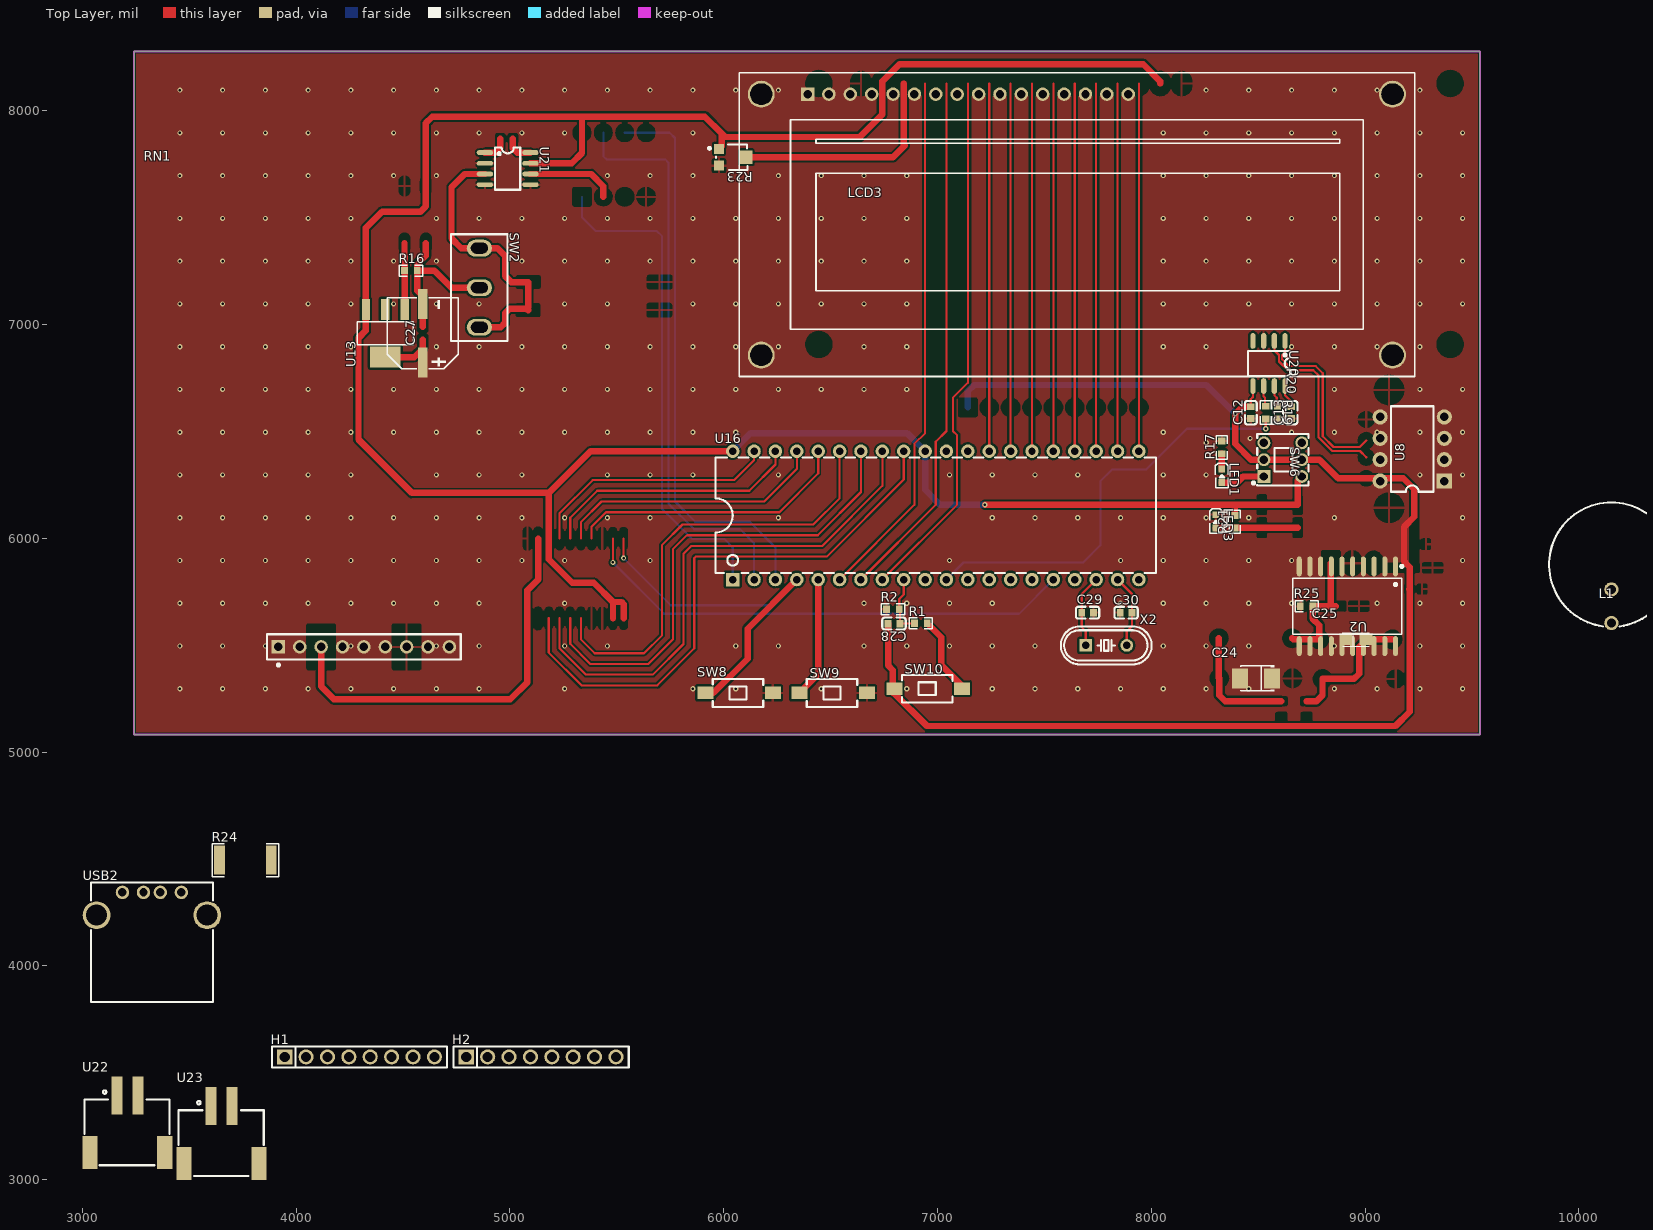
[diagram p0: Top Layer view]
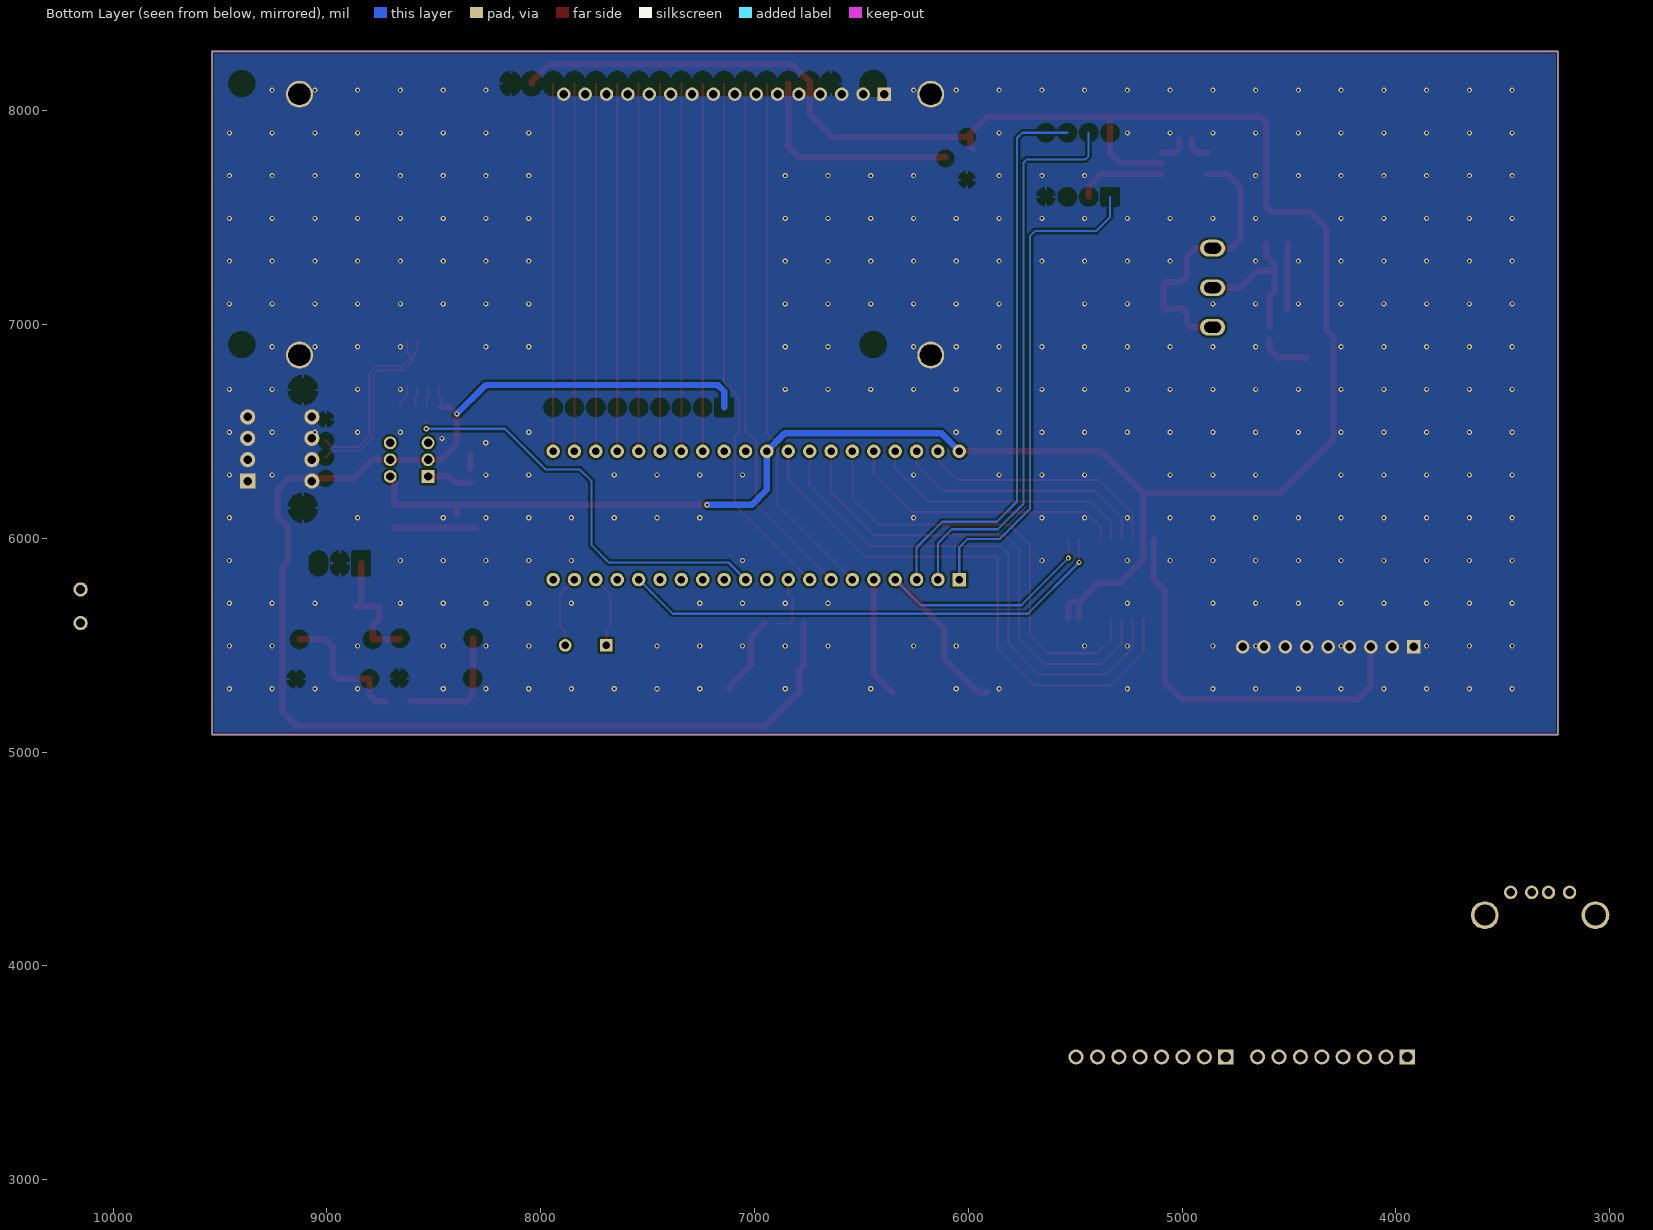
[diagram p1: Bottom Layer view, seen from below]
# Altium PCB MISC52088.pcbdoc
Units mil, origin at the board's own origin, x right, y up, seen from the top; angles counter-clockwise.
Board outline 6295 x 3195 mil, 2 copper layers (Top Layer, Bottom Layer), stack 62.206 mil thick; 40 components, 56 nets, 207 pads, 333 vias.

## Layer stack, top to bottom
Top Solder Mask Layer: solder mask 0.394, Dk 3.3
Top Layer: signal copper 1.379
Dielectric1: surface 59.449, FR4, Dk 4.5
Bottom Layer: signal copper 1.378
Bottom Solder Mask Layer: solder mask 0.394, Dk 3.3

## Board outline
3242.1,8277.43 3242.1,5082.43 9537.1,5082.43 9537.1,8277.43

## Design rules (kind name [scope] priority, off if disabled: settings)
BoardOutlineClearance copperThickness2oz_1 [All] p2 off: genericclearance=7.99 ignorepadtopadclearanceinfootprint=FALSE except(0: Arc-SplitContinuation Track-SplitContinuation SMDPad-SplitContinuation THPad-SplitContinuation Via-SplitContinuation Fill-SplitContinuation Region-SplitContinuation Poly-SplitContinuation Text-SplitContinuation Hole-SplitContinuation; 5.98: Arc-OutlineEdge Track-OutlineEdge SMDPad-OutlineEdge THPad-OutlineEdge Via-OutlineEdge Fill-OutlineEdge Region-OutlineEdge Text-OutlineEdge Hole-OutlineEdge SMDPad-CutoutEdge THPad-CutoutEdge Via-CutoutEdge Fill-CutoutEdge Region-CutoutEdge Text-CutoutEdge Hole-CutoutEdge; 10: Poly-OutlineEdge Poly-CutoutEdge; 11.81: Arc-CutoutEdge Track-CutoutEdge)
BoardOutlineClearance Plane_innerPlane_1 [All] p4 off: genericclearance=4.02 ignorepadtopadclearanceinfootprint=FALSE except(0: Arc-SplitContinuation Track-SplitContinuation SMDPad-SplitContinuation THPad-SplitContinuation Via-SplitContinuation Fill-SplitContinuation Region-SplitContinuation Poly-SplitContinuation Text-SplitContinuation Hole-SplitContinuation; 5.98: Arc-OutlineEdge Track-OutlineEdge SMDPad-OutlineEdge THPad-OutlineEdge Via-OutlineEdge Fill-OutlineEdge Region-OutlineEdge Text-OutlineEdge Hole-OutlineEdge SMDPad-CutoutEdge THPad-CutoutEdge Via-CutoutEdge Fill-CutoutEdge Region-CutoutEdge Text-CutoutEdge Hole-CutoutEdge; 10: Poly-OutlineEdge Poly-CutoutEdge; 11.81: Arc-CutoutEdge Track-CutoutEdge)
BoardOutlineClearance Copper_copperRegion_1 [All] p6 off: genericclearance=4.02 ignorepadtopadclearanceinfootprint=FALSE except(0: Arc-SplitContinuation Track-SplitContinuation SMDPad-SplitContinuation THPad-SplitContinuation Via-SplitContinuation Fill-SplitContinuation Region-SplitContinuation Poly-SplitContinuation Text-SplitContinuation Hole-SplitContinuation; 5.98: Arc-OutlineEdge Track-OutlineEdge SMDPad-OutlineEdge THPad-OutlineEdge Via-OutlineEdge Fill-OutlineEdge Region-OutlineEdge Text-OutlineEdge Hole-OutlineEdge SMDPad-CutoutEdge THPad-CutoutEdge Via-CutoutEdge Fill-CutoutEdge Region-CutoutEdge Text-CutoutEdge Hole-CutoutEdge; 10: Poly-OutlineEdge Poly-CutoutEdge; 11.81: Arc-CutoutEdge Track-CutoutEdge)
BoardOutlineClearance copperThickness1oz_1 [All] p8: genericclearance=4.02 ignorepadtopadclearanceinfootprint=FALSE except(0: Arc-SplitContinuation Track-SplitContinuation SMDPad-SplitContinuation THPad-SplitContinuation Via-SplitContinuation Fill-SplitContinuation Region-SplitContinuation Poly-SplitContinuation Text-SplitContinuation Hole-SplitContinuation; 5.98: Arc-OutlineEdge Track-OutlineEdge SMDPad-OutlineEdge THPad-OutlineEdge Via-OutlineEdge Fill-OutlineEdge Region-OutlineEdge Text-OutlineEdge Hole-OutlineEdge SMDPad-CutoutEdge THPad-CutoutEdge Via-CutoutEdge Fill-CutoutEdge Region-CutoutEdge Text-CutoutEdge Hole-CutoutEdge; 10: Poly-OutlineEdge Poly-CutoutEdge; 11.81: Arc-CutoutEdge Track-CutoutEdge)
Clearance copperThickness2oz [All] p1 off: gap=7.99 ignorepadtopadclearanceinfootprint=FALSE except(5.98: SMDPad-Track SMDPad-SMDPad THPad-Track SMDPad-THPad THPad-THPad Track-Via SMDPad-Via THPad-Via Via-Via Fill-Track Region-Track Fill-SMDPad Region-SMDPad Fill-THPad Region-THPad Fill-Via Region-Via Fill-Fill Fill-Region Region-Region Arc-SMDPad Arc-THPad Arc-Via Fill-Arc Region-Arc Arc-Arc Text-Track SMDPad-Text Text-THPad Text-Via Fill-Text Region-Text Text-Text Hole-Track Hole-SMDPad Hole-THPad Hole-Via Fill-Hole Region-Hole Hole-Arc Hole-Text; 10: Poly-Track Poly-SMDPad Poly-THPad Poly-Via Poly-Fill Poly-Region Poly-Poly Poly-Arc Poly-Text Poly-Hole; 11.81: Arc-Track Arc-Text)
Clearance Plane_innerPlane [All] p3 off: gap=4.02 ignorepadtopadclearanceinfootprint=FALSE except(5.98: SMDPad-Track SMDPad-SMDPad THPad-Track SMDPad-THPad THPad-THPad Track-Via SMDPad-Via THPad-Via Via-Via Fill-Track Region-Track Fill-SMDPad Region-SMDPad Fill-THPad Region-THPad Fill-Via Region-Via Fill-Fill Fill-Region Region-Region Arc-SMDPad Arc-THPad Arc-Via Fill-Arc Region-Arc Arc-Arc Text-Track SMDPad-Text Text-THPad Text-Via Fill-Text Region-Text Text-Text Hole-Track Hole-SMDPad Hole-THPad Hole-Via Fill-Hole Region-Hole Hole-Arc Hole-Text; 10: Poly-Track Poly-SMDPad Poly-THPad Poly-Via Poly-Fill Poly-Region Poly-Poly Poly-Arc Poly-Text Poly-Hole; 11.81: Arc-Track Arc-Text)
Clearance Copper_copperRegion [All] p5 off: gap=4.02 ignorepadtopadclearanceinfootprint=FALSE except(5.98: SMDPad-Track SMDPad-SMDPad THPad-Track SMDPad-THPad THPad-THPad Track-Via SMDPad-Via THPad-Via Via-Via Fill-Track Region-Track Fill-SMDPad Region-SMDPad Fill-THPad Region-THPad Fill-Via Region-Via Fill-Fill Fill-Region Region-Region Arc-SMDPad Arc-THPad Arc-Via Fill-Arc Region-Arc Arc-Arc Text-Track SMDPad-Text Text-THPad Text-Via Fill-Text Region-Text Text-Text Hole-Track Hole-SMDPad Hole-THPad Hole-Via Fill-Hole Region-Hole Hole-Arc Hole-Text; 10: Poly-Track Poly-SMDPad Poly-THPad Poly-Via Poly-Fill Poly-Region Poly-Poly Poly-Arc Poly-Text Poly-Hole; 11.81: Arc-Track Arc-Text)
Clearance copperThickness1oz [All] p7: gap=4.02 ignorepadtopadclearanceinfootprint=FALSE except(5.98: SMDPad-Track SMDPad-SMDPad THPad-Track SMDPad-THPad THPad-THPad Track-Via SMDPad-Via THPad-Via Via-Via Fill-Track Region-Track Fill-SMDPad Region-SMDPad Fill-THPad Region-THPad Fill-Via Region-Via Fill-Fill Fill-Region Region-Region Arc-SMDPad Arc-THPad Arc-Via Fill-Arc Region-Arc Arc-Arc Text-Track SMDPad-Text Text-THPad Text-Via Fill-Text Region-Text Text-Text Hole-Track Hole-SMDPad Hole-THPad Hole-Via Fill-Hole Region-Hole Hole-Arc Hole-Text; 10: Poly-Track Poly-SMDPad Poly-THPad Poly-Via Poly-Fill Poly-Region Poly-Poly Poly-Arc Poly-Text Poly-Hole; 11.81: Arc-Track Arc-Text)
DiffPairsRouting differentialPair [All] p1: maxlimit=6 minlimit=6 mostfreqgap=6 toplayer_minwidth=5 toplayer_prefwidth=10 toplayer_maxwidth=100 toplayer_mingap=6 toplayer_prefgap=6 toplayer_maxgap=6 bottomlayer_minwidth=5 bottomlayer_prefwidth=10 bottomlayer_maxwidth=100 bottomlayer_mingap=6 bottomlayer_prefgap=6 bottomlayer_maxgap=6 maxuncoupledlength=10
HoleToHoleClearance otherClearance [All] p1: gap=11.8 allowstackedmicrovias=TRUE
Length netLength [All] p1: minlimit=0 maxlimit=0
PasteMaskExpansion pasteMaskExpansion [All] p1: expansion=0
PlaneConnect innerPlane [All] p1: planeconnectstyle=Relief reliefexpansion=20 reliefentries=4 reliefconductorwidth=10 reliefairgap=10
PolygonConnect copperRegion [All] p1: connectstyle=Relief reliefconductorwidth=10 reliefentries=4 polygonreliefangle="90 Angle" airgapwidth=10 via.connectstyle=Relief via.reliefconductorwidth=10 via.reliefentries=4 via.polygonreliefangle="90 Angle" via.airgapwidth=10
RoutingVias viaSize [All] p1: holewidth=12.01 width=24.02 viastyle="Through Hole" minholewidth=11.81 minwidth=19.68 maxholewidth=248.03 maxwidth=393.7
SolderMaskExpansion solderMaskExpansion [IsVia] p1: expansion=-1000 istentingtop=TRUE
SolderMaskExpansion solderMaskExpansion [All] p2: expansion=2 istentingtop=FALSE
Width copperThickness2oz_2 [All] p1 off: maxlimit=100 minlimit=8 preferedwidth=10
Width copperThickness1oz_2 [All] p2: maxlimit=100 minlimit=5 preferedwidth=10

## Components (designator, comment, footprint, x,y, rotation, side; value= is the part's Value field where it differs from the comment)
C12 "0.1uF" C0603 8465.54,6587.96 r90 top
C13 "0.1uF" C0603 8655.54,6588.08 r90 top
C24 "22uF" CAP-SMD_L3.5-W2.8-R-RD 8489.27,5345.01 r0 top
C25 "100nF" CASE-A_3216 8957.1,5527.43 r0 top
C27 "100uF" CAP-SMD_BD8.1-L8.3-W8.3-LS9.3-FD 4592.12,6959.41 r90 top
C28 "47pF" C0603 6796.59,5601.57 r180 top
C29 "47pF" C0603 7702.1,5652.43 r180 top
C30 "10uF" C0603 7882.1,5652.43 r0 top
H1 "" HDR-TH_8P-P2.54-V-F-1 4296.74,3574.67 r0 top
H2 "" HDR-TH_8P-P2.54-V-F-1 5146.11,3574.67 r0 top
L1 "22uH" IND-TH_BD14.7-2P-P4.00 10152.1,5682.43 r0 top
LCD3 "HS1602A" LCD1602 7652.1,7467.43 r0 top
LED1 "" LED_0603 8330.05,6290.49 r270 top
LED3 "" LED_0603 8302.1,6077.43 r270 top
R1 "10K" R0603 6922.1,5602.43 r0 top
R2 "10K" R0603 6791.31,5668.48 r0 top
R16 "100K" R0603 4537.1,7252.43 r0 top
R17 "1K" R0603 8330.05,6425.24 r90 top
R19 "100Ω" R0603 8590.54,6588.08 r270 top
R20 "100Ω" R0603 8535.54,6588.08 r270 top
R21 "1K" R0603 8391.2,6077.73 r90 top
R23 "10kΩ" RES-ADJ-SMD_3P-L3.0-W3.8-P1.75-BR 6042.1,7782.43 r180 top
R24 "5Ω" R2512 3763,4495.45 r0 top
R25 "14kΩ" R0603 8726.82,5682.13 r0 top
RN1 "1kΩ" RES-ARRAY-TH_9P-P2.54-D1.0 4317.1,5492.43 r0 top
SW2 "SS-12D10L5" SW-TH_SS-12D10L5 4857.1,7172.43 r270 top
SW6 "5.8 ZSGT" SW-TH_5.8ZSGT 8615.54,6367.97 r270 top
SW8 "TS-1101-C-W" SW-SMD_L6.0-W3.3-LS8.0 6072.1,5277.43 r0 top
SW9 "TS-1101-C-W" SW-SMD_L6.0-W3.3-LS8.0 6512.1,5277.43 r0 top
SW10 "TS-1101-C-W" SW-SMD_L6.0-W3.3-LS8.0 6957.1,5297.43 r0 top
U2 "DAC0832LCWMX/NOPB" SOIC-20_L13.0-W7.6-P1.27-LS10.3-BL 8917.1,5682.43 r180 top
U8 "ADC0832CCN" DIP-8_L9.7-W6.4-P2.54-LS7.6-BL 9220.54,6417.97 r90 top
U13 "LT3092EST#TRPBF" SOT-223-4_L6.5-W3.5-P2.30-LS7.0-BR 4417.12,6959.41 r90 top
U16 "STC89C52RC-40I-PDIP40" DIP-40_L52.0-W13.7-P2.54-LS15.2-BL 6992.1,6107.43 r0 top
U20 "CH340N" SOP-8_L4.9-W3.9-P1.27-LS6.0-BL 8550.54,6817.97 r180 top
U21 "AD620ARZ-REEL7" SOIC-8_L5.0-W4.0-P1.27-LS6.0-BL 4989.7,7729.25 r270 top
U22 "XH2.54-2PSMD" CONN-SMD_XH2.54-2PSMD 3210.63,3260.63 r0 top
U23 "XH2.54-2PSMD" CONN-SMD_XH2.54-2PSMD 3651.58,3210.63 r0 top
USB2 "USB-231-ARY" USB-A-TH_USB-231-ARY 3325.62,4290.73 r0 top
X2 "11.0592MHz" HC-49US_L11.5-W4.5-P4.88 7789.27,5499.25 r0 top

## Footprints (in the part's own frame and the unit in brackets; to place one, negate y for a bottom-side part, rotate by r counter-clockwise, add the part's x,y. Pads: shape width x height; smd on the part's side, far side on the other; paste and mask are expansions set on the pad)
C0603 [mm]
  rect 0.8x0.9 smd: 1(-0.7,0) 2(0.7,0)
  silkscreen extent -1.39,-0.71 1.39,0.71
CAP-SMD_BD8.1-L8.3-W8.3-LS9.3-FD [mm]
  rect 3.56x1.12 smd: 1(-3.47,0) 2(3.47,0)
  silkscreen extent -4.23,-4.23 4.23,4.23
CAP-SMD_L3.5-W2.8-R-RD [mm]
  rect 1.9x2.376 smd: 1(1.899,0) 2(-1.899,0)
  silkscreen extent -1.83,-1.55 2.21,1.55
CASE-A_3216 [mil]
  rect 59.05x53.5 smd: 1(-47.24,0) 2(47.24,0)
  silkscreen extent -63,-32 63,32
CONN-SMD_XH2.54-2PSMD [mm]
  rect 1.3x4.5 smd paste+0 mask+0.05: 1(-1.25,3.4) 2(1.25,3.4)
  rect 1.8x3.9 smd paste+0 mask+0.05: 3(-4.45,-3.4) 4(4.45,-3.4)
  silkscreen extent -5.1,-4.9 5,4
DIP-8_L9.7-W6.4-P2.54-LS7.6-BL [mm]
  rect 1.8x1.8 hole 1 paste+0 mask+0.05: 1(-3.81,-3.81)
  round 1.8 hole 1 paste+0 mask+0.05: 2(-1.27,-3.81) 3(1.27,-3.81) 4(3.81,-3.81) 5(3.81,3.81) 6(1.27,3.81) 7(-1.27,3.81) 8(-3.81,3.81)
  silkscreen extent -5.08,-2.53 5.08,2.53
DIP-40_L52.0-W13.7-P2.54-LS15.2-BL [mil]
  rect 63x63 hole 35: 1(-950,-300)
  round 63 hole 35: 2(-850,-300) 3(-750,-300) 4(-650,-300) 5(-550,-300) 6(-450,-300) 7(-350,-300) 8(-250,-300) 9(-150,-300) 10(-50,-300) 11(50,-300) 12(150,-300) 13(250,-300) 14(350,-300) 15(450,-300) 16(550,-300) 17(650,-300) 18(750,-300) 19(850,-300) 20(950,-300) 21(950,300) 22(850,300) 23(750,300) 24(650,300) 25(550,300) 26(450,300) 27(350,300) 28(250,300) 29(150,300) 30(50,300) 31(-50,300) 32(-150,300) 33(-250,300) 34(-350,300) 35(-450,300) 36(-550,300) 37(-650,300) 38(-750,300) 39(-850,300) 40(-950,300)
  silkscreen extent -1030,-270 1030,270
HC-49US_L11.5-W4.5-P4.88 [mm]
  rect 1.5x1.5 hole 0.9: 1(-2.44,0)
  round 1.5 hole 0.9: 2(2.44,0)
  silkscreen extent -5.39,-2.25 5.39,2.25
HDR-TH_8P-P2.54-V-F-1 [mm]
  rect 1.8x1.8 hole 1.2: 1(-8.89,0)
  round 1.8 hole 1.2: 2(-6.35,0) 3(-3.81,0) 4(-1.27,0) 5(1.27,0) 6(3.81,0) 7(6.35,0) 8(8.89,0)
  silkscreen extent -10.41,-1.25 10.41,1.25
IND-TH_BD14.7-2P-P4.00 [mm]
  round 1.7 hole 1.1 paste+0 mask+0.05: 1(0,-2) 2(0,2)
  silkscreen extent -7.4,-2.39 7.4,12.35
LCD1602 [mm]
  round 3.2 hole 2.5 slot 2.625 at 0 deg: 0(-37.5,-15.5) 0(-37.5,15.5) 0(37.5,-15.5) 0(37.5,15.5)
  rect 1.6x1.6 hole 1: 1(-32,15.5)
  round 1.6 hole 1: 2(-29.46,15.5) 3(-26.92,15.5) 4(-24.38,15.5) 5(-21.84,15.5) 6(-19.3,15.5) 7(-16.76,15.5) 8(-14.22,15.5) 9(-11.68,15.5) 10(-9.14,15.5) 11(-6.6,15.5) 12(-4.06,15.5) 13(-1.52,15.5) 14(1.02,15.5) 15(3.56,15.5) 16(6.1,15.5)
  silkscreen extent -40.13,-18.03 40.13,18.03
LED_0603 [mil]
  rect 31.5x31.5 smd paste+0 mask+2: 1(-33.5,-0.4) 2(29.5,-0.2)
  silkscreen extent -61,-30 53,30
R0603 [mil]
  rect 31.75x34.02 smd paste-3937.01 mask+2: 1(-29.66,0) 2(29.66,0)
  silkscreen extent -55,-26 55,26
R2512 [mil]
  rect 50.49x136.06 smd paste-3937.01 mask+2: 1(-120.72,0) 2(120.72,0)
  silkscreen extent -155,-77 155,77
RES-ADJ-SMD_3P-L3.0-W3.8-P1.75-BR [mm]
  rect 1.2x1.2 smd: 1(1.625,-1) 3(1.625,1)
  rect 1.5x1.6 smd: 2(-1.625,0)
  silkscreen extent -1.75,-1.51 2.92,1.51
RES-ARRAY-TH_9P-P2.54-D1.0 [mm]
  rect 1.6x1.6 hole 1: 1(-10.16,0)
  round 1.6 hole 1: 2(-7.62,0) 3(-5.08,0) 4(-2.54,0) 5(0,0) 6(2.54,0) 7(5.08,0) 8(7.62,0) 9(10.16,0)
  silkscreen extent -11.5,-2.31 11.5,1.5
SOIC-8_L5.0-W4.0-P1.27-LS6.0-BL [mil]
  oval 22.38x76.78 smd: 1(-75,-106.5) 2(-25,-106.5) 3(25,-106.5) 4(75,-106.5) 5(75,106.5) 6(25,106.5) 7(-25,106.5) 8(-75,106.5)
  silkscreen extent -98,-59 98,59
SOIC-20_L13.0-W7.6-P1.27-LS10.3-BL [mm]
  oval 0.595x2.36 smd: 1(-5.715,-4.73) 2(-4.445,-4.73) 3(-3.175,-4.73) 4(-1.905,-4.73) 5(-0.635,-4.73) 6(0.635,-4.73) 7(1.905,-4.73) 8(3.175,-4.73) 9(4.445,-4.73) 10(5.715,-4.73) 11(5.715,4.73) 12(4.445,4.73) 13(3.175,4.73) 14(1.905,4.73) 15(0.635,4.73) 16(-0.635,4.73) 17(-1.905,4.73) 18(-3.175,4.73) 19(-4.445,4.73) 20(-5.715,4.73)
  silkscreen extent -6.61,-4.88 6.48,3.32
SOP-8_L4.9-W3.9-P1.27-LS6.0-BL [mm]
  oval 0.63x1.865 smd: 1(-1.905,-2.682) 2(-0.635,-2.682) 3(0.635,-2.682) 4(1.905,-2.682) 5(1.905,2.682) 6(0.635,2.682) 7(-0.635,2.682) 8(-1.905,2.682)
  silkscreen extent -2.5,-1.5 2.5,1.48
SOT-223-4_L6.5-W3.5-P2.30-LS7.0-BR [mm]
  rect 2.47x0.98 smd: 1(2.835,-2.3) 2(2.835,0) 3(2.835,2.3)
  rect 2.47x3.6 smd: 4(-2.835,0)
  silkscreen extent -1.37,-3.33 1.37,3.33
SW-SMD_L6.0-W3.3-LS8.0 [mm]
  rect 1.9x1.5 smd: 1(-4,0) 2(4,0)
  silkscreen extent -3.14,-1.67 2.86,1.63
SW-TH_5.8ZSGT [mm]
  rect 1.524x1.524 hole 1: 1(2,-2.25)
  round 1.524 hole 1: 2(0,-2.25) 3(-2,-2.25) 4(2,2.25) 5(0,2.25) 6(-2,2.25)
  silkscreen extent -3.05,-3.64 3.05,3.05
SW-TH_SS-12D10L5 [mm]
  oval 2x3 hole 1.3 slot 2 at 90 deg: 1(-4.7,0) 2(0,0) 3(4.7,0)
  silkscreen extent -6.35,-3.35 6.35,3.35
USB-A-TH_USB-231-ARY [mm]
  round 1.6 hole 1: 1(-3.5,1.355) 2(-1,1.355) 3(1,1.355) 4(3.5,1.355)
  round 3.3 hole 2.5: 5(-6.57,-1.355) 6(6.57,-1.355)
  silkscreen extent -7.23,-11.68 7.24,2.54

## Via types
v1: diameter 24.02, hole 12, Top Layer to Bottom Layer, 333 vias

## Nets (pads, with @x,y where several pads share a name; then routed paths per layer and width w, separated by ;. In a path a pad name is that pad's centre, name@x,y a point inside that pad or via, vN(x,y) a via of type N, cw(c..) or ccw(c..) an arc to the next point about the centre after c; other vN are vias at no path point)
5V: LED1.2 SW6.1 U23.1 | length 208.8
  Top Layer w30: LED1.2 8400.66,6260.99 8428.89,6289.23 SW6.1
$1N1971: R1.2 SW10.2 | length 372.4
  Top Layer w30: R1.2 7017.1,5537.09 7017.1,5407.43 7114.58,5309.95 SW10.2
$1N7746: LCD3.7 RN1.2 U16.28 | length 1720
  Top Layer w10: U16.28 7242.1,8127.43
$1N7754: LCD3.8 RN1.3 U16.27 | length 1720
  Top Layer w10: U16.27 7342.1,8127.43
$1N7769: LCD3.9 RN1.4 U16.26 | length 1720
  Top Layer w10: U16.26 7442.1,8127.43
$1N7777: LCD3.10 RN1.5 U16.25 | length 1720
  Top Layer w10: U16.25 7542.1,8127.43
$1N7792: LCD3.11 RN1.6 U16.24 | length 1720
  Top Layer w10: U16.24 7642.1,8127.43
$1N7807: LCD3.12 RN1.7 U16.23 | length 1720
  Top Layer w10: U16.23 7742.1,8127.43
$1N7815: LCD3.13 RN1.8 U16.22 | length 1720
  Top Layer w10: U16.22 7842.1,8127.43
$1N7830: LCD3.14 RN1.9 U16.21 | length 1720
  Top Layer w10: U16.21 7942.1,8127.43
$1N9685: C30.1 R1.1 R2.2 U16.9 | length 284.6
  Top Layer w10: U16.9 6842.1,5737.43 6820.97,5716.3 R2.2 6824.15,5665.3 6824.15,5601.57 6891.57,5601.57 R1.1
$1N13806:  | length 639.9
  Top Layer w30: 8726.16,5238.26 8772.93,5238.26 8800.84,5266.17 8800.84,5342.43 8947.1,5342.43 8972.1,5367.43 8972.1,5492.43 9007.1,5527.43 9128.36,5527.43
$1N14180:  | length 568.6
  Top Layer w30: 8315.84,5532.43 8315.84,5347.18 8318.01,5345.01 8318.01,5266.52 8346.27,5238.26 8608.05,5238.26
$1N17500: R24.1 U13.4 | length 233.7
  Top Layer w30: U13.4 4552.47,6847.8 4592.12,6887.46 4592.12,6929.75
$1N18707: C28.2 U16.18 X2.1 | length 343.9
  Top Layer w10: X2.1 7693.22,5566.32 7674.54,5584.99 7674.54,5652.43 7674.54,5739.87 U16.18
$1N18717: C29.2 U16.19 X2.2 | length 346.2
  Top Layer w10: U16.19 7909.66,5739.87 7909.66,5652.43 7909.66,5589.99 7885.34,5565.67 X2.2
$1N19281:  | length 606.9
  Top Layer w30: 8658.36,5532.43 8663.36,5527.43 8785.84,5527.43 8785.84,5593.69 8754.38,5625.16 8754.38,5682.13 8755.23,5682.98 8839.29,5682.98 ; 8839.93,5883.36 8839.93,5683.62 8839.29,5682.98 ; 8863,5682.98 8839.29,5682.98
$1N20482: R16.1 U13.1 | length 309.8
  Top Layer w30: 4507.12,7380.55 4507.12,7317.41 4507.44,7317.09 R16.1 4507.44,7158.24 4507.67,7158.01 U13.1
$1N25075: LED1.1 R17.1 | length 71.8
  Top Layer w30: LED1.1 8330.05,6324.39 R17.1
$1N27445: LCD3.3 R23.2 | length 1055.9
  Top Layer w30: R23.2 6792.1,7782.43 6847.1,7837.43 6842.1,7842.43 6842.1,8127.43
$1N30925: C13.2 U20.8 | length 109.1
  Top Layer w10: U20.8 8625.54,6668.99 8655.54,6638.99 C13.2
$1N30929: R19.1 U20.7 | length 100.8
  Top Layer w10: U20.7 8575.54,6668.99 8587.1,6657.43 8587.1,6621.19 R19.1
$1N30932: R20.1 U20.6 | length 98.8
  Top Layer w10: U20.6 8525.54,6663.99 8532.1,6657.43 8532.1,6621.19 R20.1
$1N33023:  | length 383
  Top Layer w30: 8301.9,6047.93 8303.52,6049.55 8684.28,6049.55
$1N35283: R16.2 R24.2 SW2.2 | length 731.8
  Top Layer w30: R16.2@4577.1,7252.43 4647.1,7252.43 4727.1,7172.43 SW2.2 ; 4592.12,6989.07 4592.12,7132.41 4566.76,7157.77 R16.2 4566.76,7282.09 4607.12,7322.46 4607.12,7380.55
$1N38066: R25.2 U21.1 | length 124.5
  Top Layer w30: U21.1 4933.92,7804.25 4955.04,7825.37 4955.04,7869.25
$1N38070: R25.1 U21.8 | length 134.6
  Top Layer w30: 5014.36,7869.25 5014.36,7825.17 5035.28,7804.25 U21.8
$1N38159: H1.1 H2.1 SW2.1 SW2.3 U21.3 | length 1341.7
  Top Layer w30: SW2.3 4957.06,6987.39 4977.1,7007.43 4977.1,7052.43 4998.31,7073.65 5078.8,7073.65 ; U21.3 4788.92,7704.25 4727.1,7642.43 4727.1,7402.43 4772.06,7357.47 SW2.1 4942.06,7357.47 4977.1,7322.43 4977.1,7227.43 5005.77,7198.77 5086.31,7198.77 5086.31,7081.16 5078.8,7073.65 ; 5085.01,7067.43 5078.8,7073.65
$1N38194: U8.2 U21.6 | length 414.4
  Top Layer w30: U21.6 5380.28,7704.25 5437.1,7647.43 5437.1,7597.43
$1N49753: LED3.2 R21.1
$1N51695: L1.1 U2.9 U2.11
+5V: C24.1 C25.1 C27.2 LCD3.2 LCD3.15 R21.2 SW6.4 U2.8 U2.19 U2.20 U8.8 U13.3 U16.31 U16.40 U21.7 | length 11921.1
  Top Layer w30: U21.7 5288.92,7754.25 5337.1,7802.43 5337.1,7897.43 5337.1,7972.43 ; 5482.1,5626.21 5482.1,5702.43 ; 5532.1,5626.21 5532.1,5692.43 5522.1,5702.43 5482.1,5702.43 ; 5978.12,7821.8 5990.2,7833.88 5990.2,7894.33 ; U16.40 5377.1,6407.43 5182.1,6212.43 ; v1(7222.1,6157.35) 8391.2,6157.35 ; 8042.1,8127.43 8042.1,8137.27 7961.94,8217.43 6822.26,8217.43 6742.1,8137.27 6742.1,7982.43 6637.1,7877.43 6007.1,7877.43 5990.2,7894.33 ; R21.2 8391.2,6157.35 ; SW6.4 8684.28,6269.38 8684.28,6157.35 8391.2,6157.35 ; 5182.1,6212.43 5182.1,5998.65 5182.1,5902.43 5292.1,5792.43 5392.1,5792.43 5482.1,5702.43 ; 5182.1,6212.43 4542.1,6212.43 4292.1,6462.43 4292.1,6937.43 4326.57,6971.91 U13.3 4326.57,7451.91 4402.1,7527.43 4582.1,7527.43 4607.12,7552.46 4607.12,7648.27 4607.12,7942.46 4637.1,7972.43 5337.1,7972.43 ; 5337.1,7972.43 5912.1,7972.43 5990.2,7894.33
  Bottom Layer w30: U16.40 6127.1,6492.43 6857.1,6492.43 U16.31 6942.1,6227.43 7012.18,6157.35 v1(7222.1,6157.35)
D+: U20.1 USB2.3 | length 840.4
  Top Layer w10: U20.1 8625.54,6870.87 8612.1,6857.43 8612.1,6837.43 8643.98,6805.56 8768.98,6805.56 8802.1,6772.43 8802.1,6477.43 8852.1,6427.43 8975.01,6427.43 9005.54,6457.97
D-: U20.2 USB2.2 | length 869
  Top Layer w10: U20.2 8575.54,6878.99 8597.1,6857.43 8597.1,6827.43 8638.18,6786.35 8758.18,6786.35 8782.1,6762.43 8782.1,6472.43 8846.12,6408.42 8976.35,6408.42 9005.54,6379.22
GND: C12.1 C13.1 C24.2 C25.2 C27.1 C28.1 C29.1 H1.8 H2.8 L1.2 LCD3.1 LCD3.16 LED3.1 R2.1 R17.2 R23.1 R23.3 SW8.2 SW9.2 U2.3 U2.10 U2.17 U2.18 U8.4 U20.3 U21.2 U21.4 U21.5 U22.2 U23.2 USB2.4 USB2.5 USB2.6
  other v1: 3456.2,5296.53 3656.2,5296.53 3856.2,5296.53 4056.2,5296.53 4256.2,5296.53 4456.2,5296.53 4656.2,5296.53 4856.2,5296.53 5256.2,5296.53 5856.2,5296.53 6056.2,5296.53 6456.2,5296.53 6856.2,5296.53 7256.2,5296.53 7456.2,5296.53 7656.2,5296.53 7856.2,5296.53 8056.2,5296.53 8256.2,5296.53 8456.2,5296.53 8856.2,5296.53 9256.2,5296.53 9456.2,5296.53 3456.2,5496.53 3656.2,5496.53 3856.2,5496.53 4256.2,5496.53 4656.2,5496.53 4856.2,5496.53 5256.2,5496.53 5456.2,5496.53 6056.2,5496.53 6256.2,5496.53 6656.2,5496.53 6856.2,5496.53 7056.2,5496.53 7256.2,5496.53 7456.2,5496.53 8056.2,5496.53 8256.2,5496.53 8456.2,5496.53 8856.2,5496.53 9256.2,5496.53 9456.2,5496.53 3456.2,5696.53 3656.2,5696.53 3856.2,5696.53 4056.2,5696.53 4256.2,5696.53 4456.2,5696.53 4656.2,5696.53 4856.2,5696.53 5256.2,5696.53 6656.2,5696.53 6856.2,5696.53 7056.2,5696.53 7256.2,5696.53 7856.2,5696.53 8056.2,5696.53 8256.2,5696.53 8456.2,5696.53 8656.2,5696.53 9056.2,5696.53 9256.2,5696.53 9456.2,5696.53 3456.2,5896.53 3656.2,5896.53 3856.2,5896.53 4056.2,5896.53 4256.2,5896.53 4456.2,5896.53 4656.2,5896.53 4856.2,5896.53 5056.2,5896.53 5256.2,5896.53 5656.2,5896.53 7056.2,5896.53 7856.2,5896.53 8056.2,5896.53 8256.2,5896.53 8456.2,5896.53 8656.2,5896.53 9456.2,5896.53 3456.2,6096.53 3656.2,6096.53 3856.2,6096.53 4056.2,6096.53 4256.2,6096.53 4456.2,6096.53 4656.2,6096.53 4856.2,6096.53 5056.2,6096.53 5256.2,6096.53 5456.2,6096.53 5656.2,6096.53 6256.2,6096.53 7256.2,6096.53 7456.2,6096.53 7656.2,6096.53 7856.2,6096.53 8056.2,6096.53 8256.2,6096.53 8456.2,6096.53 8856.2,6096.53 9456.2,6096.53 3456.2,6296.53 3656.2,6296.53 3856.2,6296.53 4056.2,6296.53 4256.2,6296.53 4656.2,6296.53 4856.2,6296.53 5056.2,6296.53 5456.2,6296.53 5656.2,6296.53 5856.2,6296.53 6256.2,6296.53 7056.2,6296.53 7256.2,6296.53 7456.2,6296.53 7656.2,6296.53 8056.2,6296.53 8256.2,6296.53 9256.2,6296.53 9456.2,6296.53 8257.1,6447.43 8462.1,6467.43 3456.2,6496.53 3656.2,6496.53 3856.2,6496.53 4056.2,6496.53 4256.2,6496.53 4456.2,6496.53 4656.2,6496.53 4856.2,6496.53 5056.2,6496.53 5256.2,6496.53 5456.2,6496.53 5656.2,6496.53 5856.2,6496.53 6056.2,6496.53 8056.2,6496.53 8656.2,6496.53 8856.2,6496.53 9056.2,6496.53 9256.2,6496.53 9456.2,6496.53 3456.2,6696.53 3656.2,6696.53 3856.2,6696.53 4056.2,6696.53 4256.2,6696.53 4456.2,6696.53 4656.2,6696.53 4856.2,6696.53 5056.2,6696.53 5256.2,6696.53 5456.2,6696.53 5656.2,6696.53 5856.2,6696.53 6056.2,6696.53 6256.2,6696.53 6456.2,6696.53 6656.2,6696.53 6856.2,6696.53 8656.2,6696.53 8856.2,6696.53 9256.2,6696.53 9456.2,6696.53 3456.2,6896.53 3656.2,6896.53 3856.2,6896.53 4056.2,6896.53 4256.2,6896.53 4656.2,6896.53 4856.2,6896.53 5056.2,6896.53 5256.2,6896.53 5456.2,6896.53 5656.2,6896.53 5856.2,6896.53 6056.2,6896.53 6256.2,6896.53 6656.2,6896.53 6856.2,6896.53 8056.2,6896.53 8256.2,6896.53 8656.2,6896.53 8856.2,6896.53 9056.2,6896.53 9256.2,6896.53 3456.2,7096.53 3656.2,7096.53 3856.2,7096.53 4056.2,7096.53 4256.2,7096.53 4456.2,7096.53 4656.2,7096.53 4856.2,7096.53 5256.2,7096.53 5456.2,7096.53 5856.2,7096.53 6056.2,7096.53 6256.2,7096.53 6456.2,7096.53 6656.2,7096.53 6856.2,7096.53 8056.2,7096.53 8256.2,7096.53 8456.2,7096.53 8656.2,7096.53 8856.2,7096.53 9056.2,7096.53 9256.2,7096.53 9456.2,7096.53 3456.2,7296.53 3656.2,7296.53 3856.2,7296.53 4056.2,7296.53 4256.2,7296.53 4456.2,7296.53 4656.2,7296.53 5056.2,7296.53 5256.2,7296.53 5456.2,7296.53 5656.2,7296.53 5856.2,7296.53 6056.2,7296.53 6256.2,7296.53 6456.2,7296.53 6656.2,7296.53 6856.2,7296.53 8056.2,7296.53 8256.2,7296.53 8456.2,7296.53 8656.2,7296.53 8856.2,7296.53 9056.2,7296.53 9256.2,7296.53 9456.2,7296.53 3456.2,7496.53 3656.2,7496.53 3856.2,7496.53 4056.2,7496.53 4256.2,7496.53 4656.2,7496.53 4856.2,7496.53 5056.2,7496.53 5256.2,7496.53 5456.2,7496.53 5656.2,7496.53 5856.2,7496.53 6056.2,7496.53 6256.2,7496.53 6456.2,7496.53 6656.2,7496.53 6856.2,7496.53 8056.2,7496.53 8256.2,7496.53 8456.2,7496.53 8656.2,7496.53 9056.2,7496.53 9256.2,7496.53 9456.2,7496.53 3456.2,7696.53 3656.2,7696.53 3856.2,7696.53 4056.2,7696.53 4256.2,7696.53 4456.2,7696.53 4656.2,7696.53 5456.2,7696.53 5656.2,7696.53 5856.2,7696.53 6256.2,7696.53 6456.2,7696.53 6656.2,7696.53 6856.2,7696.53 8056.2,7696.53 8256.2,7696.53 8456.2,7696.53 8656.2,7696.53 8856.2,7696.53 9056.2,7696.53 9256.2,7696.53 9456.2,7696.53 3456.2,7896.53 3656.2,7896.53 3856.2,7896.53 4056.2,7896.53 4256.2,7896.53 4456.2,7896.53 4656.2,7896.53 4856.2,7896.53 5056.2,7896.53 5256.2,7896.53 5856.2,7896.53 8056.2,7896.53 8256.2,7896.53 8456.2,7896.53 8656.2,7896.53 8856.2,7896.53 9056.2,7896.53 9256.2,7896.53 9456.2,7896.53 3456.2,8096.53 3656.2,8096.53 3856.2,8096.53 4056.2,8096.53 4256.2,8096.53 4456.2,8096.53 4656.2,8096.53 4856.2,8096.53 5056.2,8096.53 5256.2,8096.53 5456.2,8096.53 5656.2,8096.53 5856.2,8096.53 6056.2,8096.53 6256.2,8096.53 8256.2,8096.53 8456.2,8096.53 8656.2,8096.53 8856.2,8096.53 9056.2,8096.53 9256.2,8096.53
P0.0: U2.7 U16.39 | length 1173.1
  Top Layer w10: 5232.1,5998.65 5232.1,6117.24 5387.29,6272.43 6048.6,6272.43 6142.1,6365.93 U16.39
P0.1: U2.6 U16.38 | length 1223.1
  Top Layer w10: 5282.1,5998.65 5282.1,6096.53 5408,6222.43 6119.31,6222.43 6242.1,6345.22 U16.38
P0.2: U2.5 U16.37 | length 1273.1
  Top Layer w10: 5332.1,5998.65 5332.1,6075.82 5428.71,6172.43 6190.02,6172.43 6342.1,6324.51 U16.37
P0.3: U2.4 U16.36 | length 1323.1
  Top Layer w10: 5382.1,5998.65 5382.1,6055.11 5449.42,6122.43 6260.73,6122.43 6442.1,6303.8 U16.36
P0.4: U2.16 U16.35 | length 2103.3
  Top Layer w10: 5332.1,5626.21 5332.1,5527.43 5397.1,5462.43 5627.1,5462.43 5712.1,5547.43 5712.1,5969.56 5807.04,6064.5 6419.17,6064.5 6542.1,6187.43 U16.35
P0.5: U2.15 U16.34 | length 2289.7
  Top Layer w10: 5282.1,5626.21 5282.1,5506.72 5376.39,5412.43 5647.81,5412.43 5762.1,5526.72 5762.1,5948.85 5827.75,6014.5 6439.88,6014.5 6642.1,6216.72 U16.34
P0.6: U2.14 U16.33 | length 2476.1
  Top Layer w10: 5232.1,5626.21 5232.1,5486.01 5355.68,5362.43 5668.52,5362.43 5812.1,5506.01 5812.1,5928.14 5848.46,5964.5 6460.59,5964.5 6742.1,6246.01 U16.33
P0.7: U2.13 U16.32 | length 2662.5
  Top Layer w10: 5182.1,5626.21 5182.1,5465.3 5334.97,5312.43 5689.23,5312.43 5862.1,5485.3 5862.1,5907.43 5869.17,5914.5 6481.3,5914.5 6842.1,6275.3 U16.32
P1.0: U8.1 U16.1 | length 2336.8
  Bottom Layer w10: 5337.1,7597.43 5337.1,7502.43 5402.1,7437.43 5687.1,7437.43 5712.1,7412.43 5712.1,6137.43 5852.1,5997.43 6002.1,5997.43 6042.1,5957.43 U16.1
P1.1: U8.7 U16.2 | length 2669.1
  Bottom Layer w10: 5437.1,7897.43 5437.1,7787.43 5452.1,7772.43 5727.1,7772.43 5742.1,7757.43 5742.1,6162.43 5862.1,6042.43 6077.1,6042.43 6142.1,5977.43 U16.2
P1.2: U8.5 U8.6 U16.3 | length 2654.4
  Bottom Layer w10: 5537.1,7897.43 5637.1,7897.43 5747.1,7897.43 5772.1,7872.43 5772.1,6172.43 5867.1,6077.43 6122.1,6077.43 6242.1,5957.43 U16.3
P1.3: SW8.1 U2.1 U16.4 | length 1771.1
  Top Layer w10: v1(5532.1,5907.43) 5532.1,5998.65
  Top Layer w30: SW8.1 5952.1,5277.43 6112.1,5437.43 6112.1,5577.43 U16.4
  Bottom Layer w10: v1(5532.1,5907.43) 5752.1,5687.43 6222.1,5687.43 U16.4
P1.4: SW9.1 U16.5 | length 566.2
  Top Layer w30: SW9.1 6442.1,5364.91 U16.5
P1.5: LCD3.4 U16.6 | length 2485.7
  Top Layer w10: U16.6 6892.1,6157.43 6892.1,6442.43 6942.1,6492.43 6942.1,8127.43
P1.6: LCD3.5 U16.7 | length 2485.7
  Top Layer w10: U16.7 6992.1,6157.43 6992.1,6452.43 7042.1,6502.43 7042.1,8127.43
P1.7: LCD3.6 U16.8 | length 2502.3
  Top Layer w10: U16.8 7092.1,6157.43 7092.1,6482.43 7072.1,6502.43 7072.1,6657.43 7142.1,6727.43 7142.1,8127.43
P3.0: U16.10
P3.1: R20.2 U16.11 | length 2007.2
  Top Layer w10: v1(8535.54,6512.43) R20.2
  Bottom Layer w10: U16.11 7121.98,5887.32 7681.98,5887.32 7762.1,5967.43 7762.1,6267.43 7817.1,6322.43 7977.1,6322.43 8167.1,6512.43 v1(8535.54,6512.43)
P3.6: U2.2 U16.16 | length 2336.9
  Top Layer w10: v1(5482.1,5887.43) 5482.1,5998.65
  Bottom Layer w10: v1(5482.1,5887.43) 5722.1,5647.43 7382.1,5647.43 U16.16
P.03: R19.2
VCC: C12.2 C30.2 RN1.1 SW6.2 SW6.5 SW10.1 U20.5 U22.1 USB2.1 | length 8461.6
  Top Layer w10: C12.2 8465.54,6650.88 8475.54,6660.87 U20.5
  Top Layer w30: 4117.1,5492.43 4117.1,5307.43 4177.1,5247.43 5002.1,5247.43 5082.1,5327.43 5082.1,5757.43 5132.1,5807.43 5132.1,5998.65 ; 6769.03,5601.57 6769.03,5405.51 6791.19,5383.34 6791.19,5278.48 6794.53,5278.48 6950.58,5122.43 9142.1,5122.43 9208.4,5188.73 9208.4,5763.39 ; C12.2 8425.19,6615.52 v1(8392.1,6582.43) 8392.1,6442.43 8466.57,6367.97 SW6.2 SW6.5 8786.57,6367.97 8873.74,6280.79 9005.54,6280.79 9178.74,6280.79 9229.54,6229.99 9229.54,6100.62 9182.1,6053.18 9182.1,5891.69 9208.4,5865.39 9208.4,5763.39 ; 9207.44,5762.43 9208.4,5763.39
  Bottom Layer w30: 7142.1,6612.43 7142.1,6687.43 7172.1,6717.43 8257.1,6717.43 v1(8392.1,6582.43)
  other v1: 9056.2,5296.53
pads on no net: H1.2 H1.3 H1.4 H1.5 H1.6 H1.7 H2.2 H2.3 H2.4 H2.5 H2.6 H2.7 LCD3.0 SW6.3 SW6.6 U2.12 U8.3 U13.2 U16.12 U16.13 U16.14 U16.15 U16.17 U16.20 U16.29 U16.30 U20.4 U22.3 U22.4 U23.3 U23.4
copper on no net:
  other v1: 8856.2,7496.53

## Polygon pours and split planes (outlines as drawn)
GND on Top Layer (solid, remove dead copper, pour order 0): 3012.1,8757.43 3012.1,4832.43 9907.1,4832.43 9907.1,8757.43
GND on Bottom Layer (solid, remove dead copper, pour order 2): 3002.1,8502.43 3002.1,4772.43 9832.1,4772.43 9832.1,8502.43

## Keep-outs
Board Outline Layer:
  the board outline again, w10